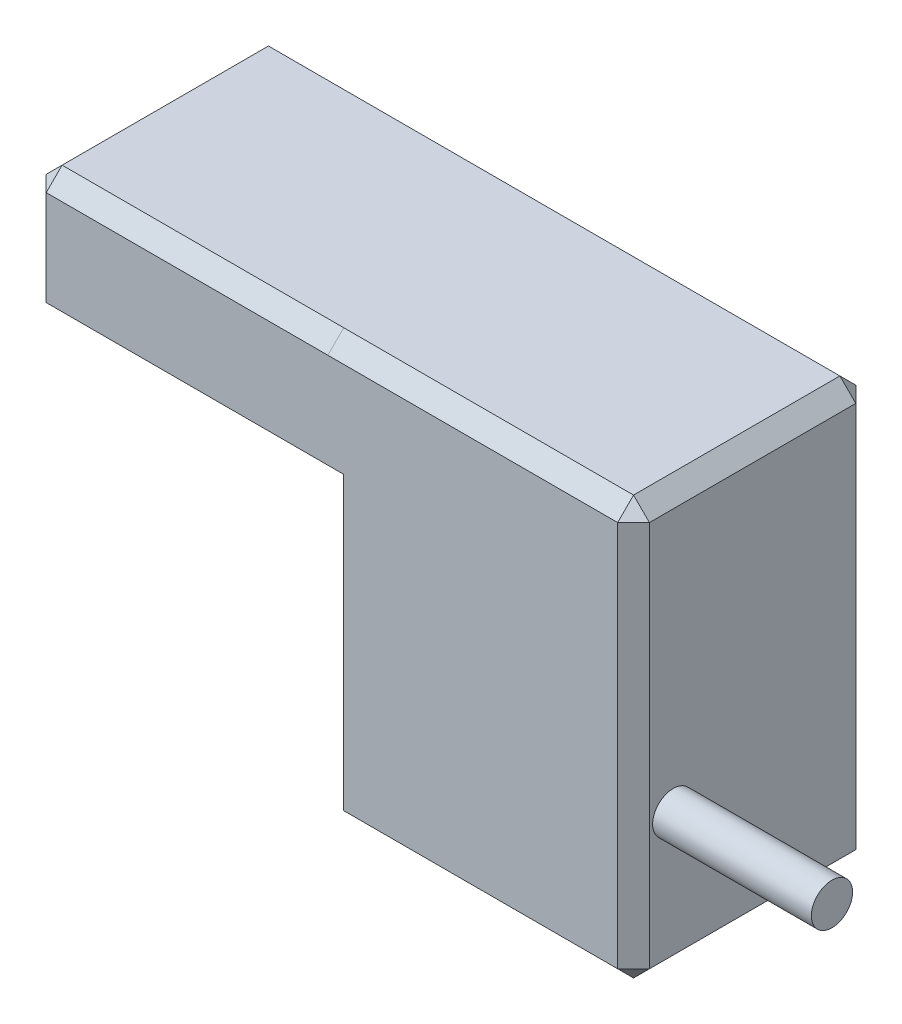
from build123d import *

# Parameters (mm, degrees)
BOSS_EXTRUDE1_DEPTH = 7.5
SKETCH3_R           = 1.3
BOSS_EXTRUDE2_DEPTH = 10
CHAMFER1_SIZE       = 1


with BuildPart() as part:
    # Model → Boss-Extrude1 (new, symmetric)
    with BuildSketch(Plane.XY):
        Polygon((-51.414562431, 5.775101607), (-51.414562431, 20.775101607), (-70.671536853, 20.775099073), (-89.414562431, 20.775100292), (-89.414562431, 15.775100292), (-89.414562431, 12.775100292), (-70.671536853, 12.775100292), (-70.671536853, 5.775101607), (-70.671536853, -5.572423542), (-51.414562431, -5.572423542), align=None)
    extrude(amount=BOSS_EXTRUDE1_DEPTH, both=True)

    # Sketch3 → Boss-Extrude2 (add)
    with BuildSketch(Plane(origin=(-51.414562431, 0, 0), x_dir=(0, 0, -1), z_dir=(1, 0, 0))):
        with Locations(Location((-5, 3.217576458, 0), (0, 0, 270))):
            Circle(SKETCH3_R)
    extrude(amount=BOSS_EXTRUDE2_DEPTH)

    # Chamfer1
    chamfer1_edges = [part.edges().sort_by_distance(p)[0] for p in [
        (-80.043049642, 20.775099682, -7.5),
        (-61.043049642, 20.77510034, -7.5),
        (-51.414562431, 7.601339033, -7.5),
        (-61.043049642, -5.572423542, -7.5),
        (-70.671536853, 3.601338375, -7.5),
        (-80.043049642, 12.775100292, -7.5),
        (-61.043049642, -5.572423542, 7.5),
        (-51.414562431, 7.601339033, 7.5),
        (-89.414562431, 12.775100292, 0),
        (-89.414562431, 20.775100292, 0),
        (-51.414562431, 20.775101607, 0),
        (-51.414562431, -5.572423542, 0),
        (-70.671536853, -5.572423542, 0),
        (-61.043049642, 20.77510034, 7.5),
        (-80.043049642, 20.775099682, 7.5),
        (-89.414562431, 16.775100292, 7.5),
        (-80.043049642, 12.775100292, 7.5),
        (-70.671536853, 3.601338375, 7.5),
        (-89.414562431, 16.775100292, -7.5),
    ]]
    chamfer(chamfer1_edges, length=CHAMFER1_SIZE)


solid = part.part
